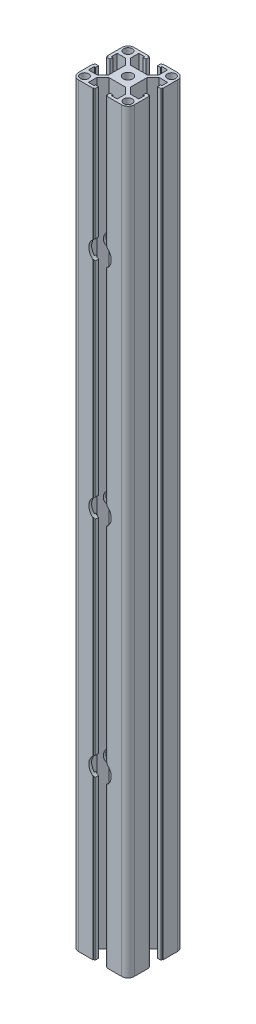
from build123d import *

# Parameters (mm, degrees)
SKETCH16_R                   = 3.4
SKETCH16_R_2                 = 3
MEMBER_1_DEPTH               = 540
HOLE_WIZARD_M8_1_D           = 9
HOLE_WIZARD_M8_1_CBORE_D     = 16
HOLE_WIZARD_M8_1_CBORE_DEPTH = 12.3


with BuildPart() as part:
    # Sketch16 → Member 1 (new body)
    with BuildSketch(Plane(origin=(0, 0, 0), x_dir=(-1, 0, 0), z_dir=(0, 1, 0))):
        with BuildLine():
            Line((-5.1, 20), (-5.1, 19.5))
            Line((-5.1, 19.5), (-4.1, 19.5))
            Line((-4.1, 19.5), (-4.1, 17))
            Line((-4.1, 17), (-6.1, 17))
            Line((-6.1, 17), (-6.1, 18))
            Line((-6.1, 18), (-10.3, 18))
            Line((-10.3, 18), (-10.3, 12))
            Line((-10.3, 12), (-6, 7.7))
            Line((-6, 7.7), (6, 7.7))
            Line((6, 7.7), (10.3, 12))
            Line((10.3, 12), (10.3, 18))
            Line((10.3, 18), (6.1, 18))
            Line((6.1, 18), (6.1, 17))
            Line((6.1, 17), (4.1, 17))
            Line((4.1, 17), (4.1, 19.5))
            Line((4.1, 19.5), (5.1, 19.5))
            Line((5.1, 19.5), (5.1, 20))
            Line((5.1, 20), (15.5, 20))
            ThreePointArc((15.5, 20), (18.681980515, 18.681980515), (20, 15.5))
            Line((20, 15.5), (20, 5.1))
            Line((20, 5.1), (19.5, 5.1))
            Line((19.5, 5.1), (19.5, 4.1))
            Line((19.5, 4.1), (17, 4.1))
            Line((17, 4.1), (17, 6.1))
            Line((17, 6.1), (18, 6.1))
            Line((18, 6.1), (18, 10.3))
            Line((18, 10.3), (12, 10.3))
            Line((12, 10.3), (7.7, 6))
            Line((7.7, 6), (7.7, -6))
            Line((7.7, -6), (12, -10.3))
            Line((12, -10.3), (18, -10.3))
            Line((18, -10.3), (18, -6.1))
            Line((18, -6.1), (17, -6.1))
            Line((17, -6.1), (17, -4.1))
            Line((17, -4.1), (19.5, -4.1))
            Line((19.5, -4.1), (19.5, -5.1))
            Line((19.5, -5.1), (20, -5.1))
            Line((20, -5.1), (20, -15.5))
            ThreePointArc((20, -15.5), (18.681980515, -18.681980515), (15.5, -20))
            Line((15.5, -20), (5.1, -20))
            Line((5.1, -20), (5.1, -19.5))
            Line((5.1, -19.5), (4.1, -19.5))
            Line((4.1, -19.5), (4.1, -17))
            Line((4.1, -17), (6.1, -17))
            Line((6.1, -17), (6.1, -18))
            Line((6.1, -18), (10.3, -18))
            Line((10.3, -18), (10.3, -12))
            Line((10.3, -12), (6, -7.7))
            Line((6, -7.7), (-6, -7.7))
            Line((-6, -7.7), (-10.3, -12))
            Line((-10.3, -12), (-10.3, -18))
            Line((-10.3, -18), (-6.1, -18))
            Line((-6.1, -18), (-6.1, -17))
            Line((-6.1, -17), (-4.1, -17))
            Line((-4.1, -17), (-4.1, -19.5))
            Line((-4.1, -19.5), (-5.1, -19.5))
            Line((-5.1, -19.5), (-5.1, -20))
            Line((-5.1, -20), (-15.5, -20))
            ThreePointArc((-15.5, -20), (-18.681980515, -18.681980515), (-20, -15.5))
            Line((-20, -15.5), (-20, -5.1))
            Line((-20, -5.1), (-19.5, -5.1))
            Line((-19.5, -5.1), (-19.5, -4.1))
            Line((-19.5, -4.1), (-17, -4.1))
            Line((-17, -4.1), (-17, -6.1))
            Line((-17, -6.1), (-18, -6.1))
            Line((-18, -6.1), (-18, -10.3))
            Line((-18, -10.3), (-12, -10.3))
            Line((-12, -10.3), (-7.7, -6))
            Line((-7.7, -6), (-7.7, 6))
            Line((-7.7, 6), (-12, 10.3))
            Line((-12, 10.3), (-18, 10.3))
            Line((-18, 10.3), (-18, 6.1))
            Line((-18, 6.1), (-17, 6.1))
            Line((-17, 6.1), (-17, 4.1))
            Line((-17, 4.1), (-19.5, 4.1))
            Line((-19.5, 4.1), (-19.5, 5.1))
            Line((-19.5, 5.1), (-20, 5.1))
            Line((-20, 5.1), (-20, 15.5))
            ThreePointArc((-20, 15.5), (-18.681980515, 18.681980515), (-15.5, 20))
            Line((-15.5, 20), (-5.1, 20))
        make_face()
        Circle(SKETCH16_R, mode=Mode.SUBTRACT)
        with Locations((-15.556349186, 15.556349186)):
            Circle(SKETCH16_R_2, mode=Mode.SUBTRACT)
        with Locations((15.556349186, 15.556349186)):
            Circle(SKETCH16_R_2, mode=Mode.SUBTRACT)
        with Locations((15.556349186, -15.556349186)):
            Circle(SKETCH16_R_2, mode=Mode.SUBTRACT)
        with Locations((-15.556349186, -15.556349186)):
            Circle(SKETCH16_R_2, mode=Mode.SUBTRACT)
    extrude(amount=MEMBER_1_DEPTH)

    # M8 六角凹头螺钉的柱形沉头孔1 (through all)
    with Locations(Plane(origin=(9.58186976, -44.093066006, 20), x_dir=(-1, 0, 0), z_dir=(0, 0, 1))):
        with Locations((9.58186976, -164.093066006), (9.58186976, -324.093066006), (9.58186976, -484.093066006)):
            CounterBoreHole(HOLE_WIZARD_M8_1_D / 2, HOLE_WIZARD_M8_1_CBORE_D / 2, HOLE_WIZARD_M8_1_CBORE_DEPTH)


solid = part.part
